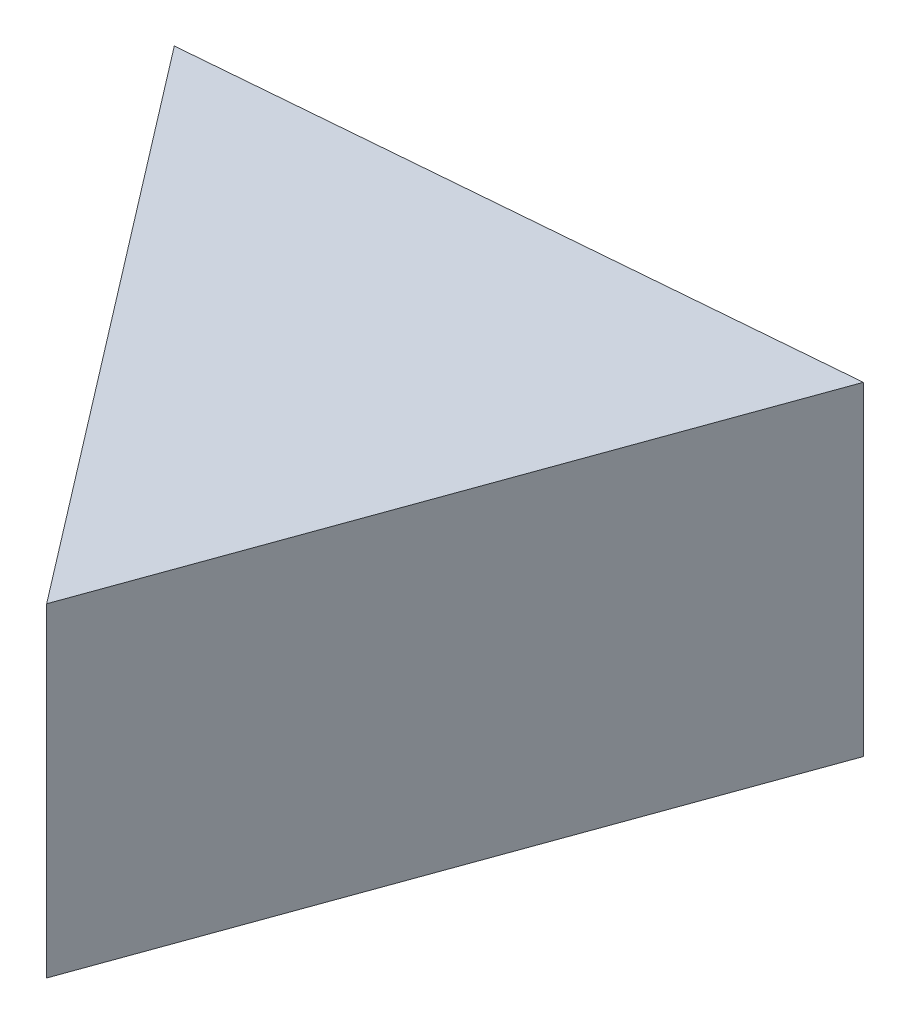
SolidWorks part; units mm, degrees
material "A-玻璃纤维"
ref_plane "Front Plane" through (0, 0, 0) normal (0, 0, 1) x (1, 0, 0)
ref_plane "Top Plane" through (0, 0, 0) normal (0, 1, 0) x (1, 0, 0)
ref_plane "Right Plane" through (0, 0, 0) normal (1, 0, 0) x (0, 0, -1)
sketch "Sketch1" plane through (0, 0, 0) normal (0, 1, 0) x (1, 0, 0)
  line L0 (0, 0) -> (-24.9127, -2.0873)
  line L1 (-24.9127, -2.0873) -> (-8.4863, -23.5156)
  line L2 (-8.4863, -23.5156) -> (0, 0)
  dimension "D1" = 25
  dimension "D2" = 25
  dimension "D3" = 27
extrude "Boss-Extrude1" add sketch "Sketch1" along normal blind 12.7
